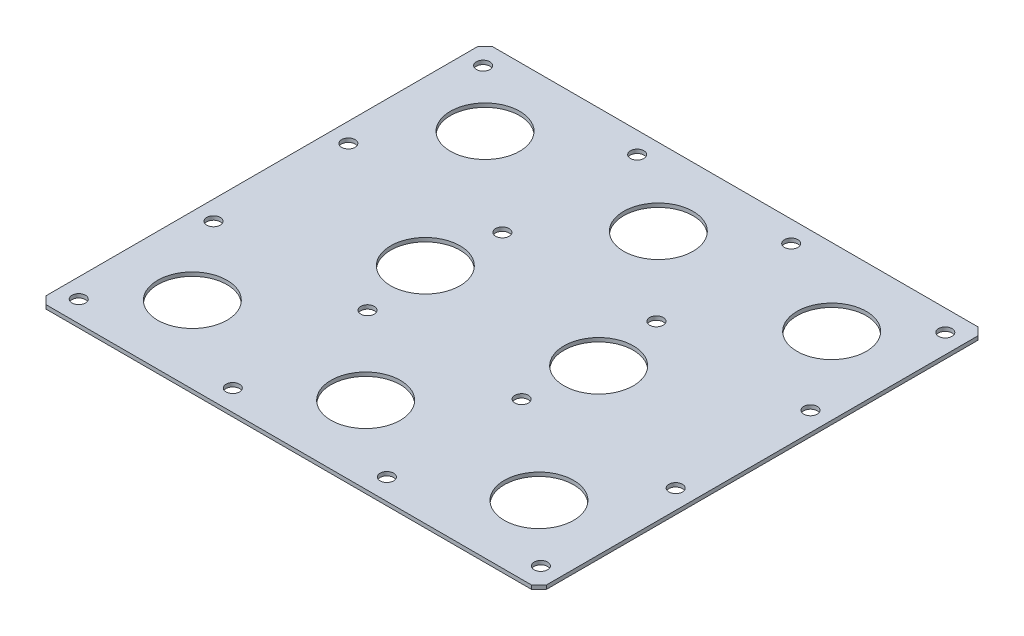
SolidWorks part; units mm, degrees
ref_plane "Front Plane" through (0, 0, 0) normal (0, 0, 1) x (1, 0, 0)
ref_plane "Top Plane" through (0, 0, 0) normal (0, 1, 0) x (1, 0, 0)
ref_plane "Right Plane" through (0, 0, 0) normal (1, 0, 0) x (0, 0, -1)
sketch "Sketch1" plane through (0, 0, 0) normal (0, 1, 0) x (1, 0, 0)
  line L1 (-65, -58) -> (65, -58)
  line L2 (-65, -58) -> (-65, 58)
  line L3 (-65, 58) -> (65, 58)
  line L4 (65, -58) -> (65, 58)
  line L5 (-65, -58) -> (65, 58) construction
  line L6 (-65, 58) -> (65, -58) construction
  point P0 (0, 0)
  dimension "D1" = 116
  dimension "D2" = 130
extrude "Boss-Extrude1" add sketch "Sketch1" along normal blind 1
sketch "Sketch2" plane through (0, 1, 0) normal (0, 1, 0) x (1, 0, 0)
  line L0 (65, -58) -> (65, 58) construction
  line L1 (-65, -58) -> (65, -58) construction
  circle A0 centre (45, -38) radius 9
  dimension "D1" = 20
  dimension "D2" = 20
  dimension "D3" = 18
extrude "Cut-Extrude1" cut sketch "Sketch2" against normal through all
pattern_linear "LPattern1" count 3 spacing 38 along (0, 0, -1) count 5 spacing 22.5 along (-1, 0, 0) skipping (0, 1), (0, 3), (1, 0), (1, 2), (1, 4), (2, 1), (2, 3) of "Cut-Extrude1"
chamfer "Chamfer1" distance 2 angle 45 4 edges at (65, 0.5, -58) (-65, 0.5, -58) (-65, 0.5, 58) (65, 0.5, 58)
hole_wizard "Ø3.5 (3.5) Diameter Hole1" positions "Sketch4" profile "Sketch3" hole size "Ø3.5" standard "Gb" end condition through all
sketch "Sketch4" plane through (0, 1, 0) normal (0, 1, 0) x (1, 0, 0)
  line L0 (-63, -58) -> (63, -58) construction
  line L1 (65, -56) -> (65, 56) construction
  point P0 (60, -52.5)
  dimension "D1" = 5.5
  dimension "D2" = 5
sketch "Sketch3" plane through (60, 1, 52.5) normal (1, 0, 0) x (0, 0, 1)
  line L0 (0, 0) -> (0, 1)
  line L1 (0, 1) -> (1.75, 1)
  line L2 (1.75, 1) -> (1.75, 0)
  line L5 (1.75, 0) -> (0, 0)
  line L11 (0, -6.35) -> (0, 107.95) construction
  dimension "通孔孔直径" = 3.5
  dimension "通孔孔深度" = 1
pattern_linear "LPattern2" count 4 spacing 40 along (-1, 0, 0) count 4 spacing 35 along (0, 0, -1) of "Ø3.5 (3.5) Diameter Hole1"
